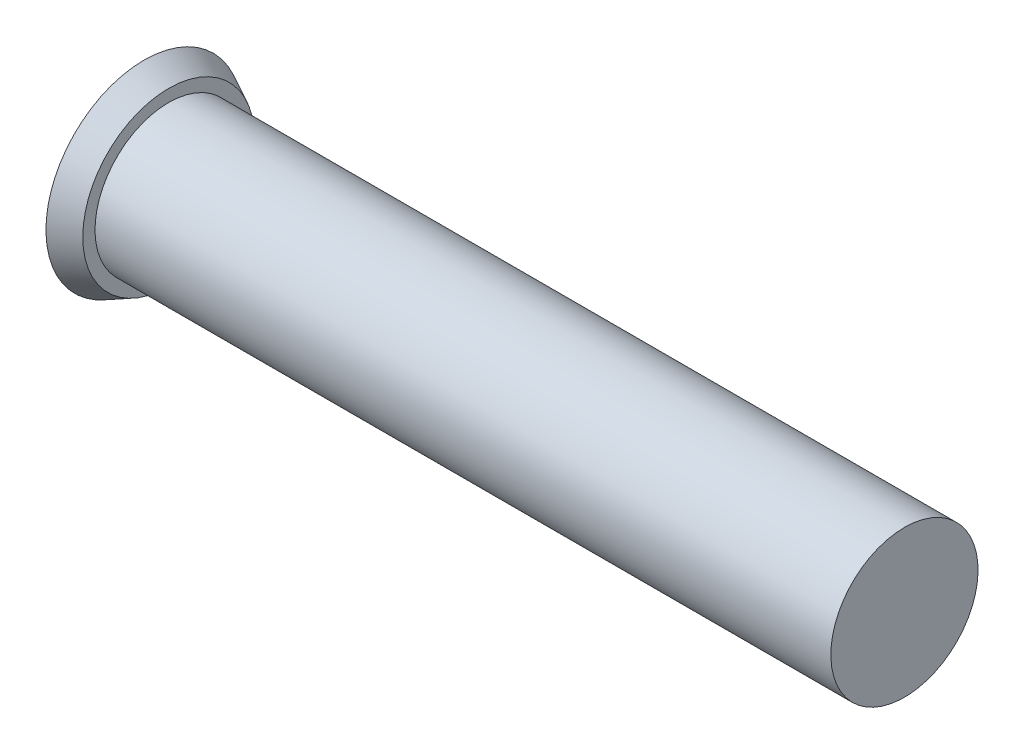
SolidWorks part; units mm, degrees
ref_plane "Front Plane" through (0, 0, 0) normal (0, 0, 1) x (1, 0, 0)
ref_plane "Top Plane" through (0, 0, 0) normal (0, 1, 0) x (1, 0, 0)
ref_plane "Right Plane" through (0, 0, 0) normal (1, 0, 0) x (0, 0, -1)
other "Configuration Table"
sketch "Sketch1" plane through (0, 0, 0) normal (0, 0, 1) x (1, 0, 0)
  line L0 (0, 0) -> (0, 4)
  line L1 (0, 4) -> (1, 3.5)
  line L2 (1, 3.5) -> (1, 3)
  line L3 (1, 3) -> (31, 3)
  line L4 (31, 3) -> (31, 0)
  line L5 (31, 0) -> (0, 0) construction
  line L6 (0, 0) -> (31, 0)
  dimension "D1" = 6
  dimension "D2" = 8
  dimension "D3" = 7
  dimension "D4" = 1
  dimension "D5" = 31
revolve "Revolve1" add sketch "Sketch1" angle 360 about L5
